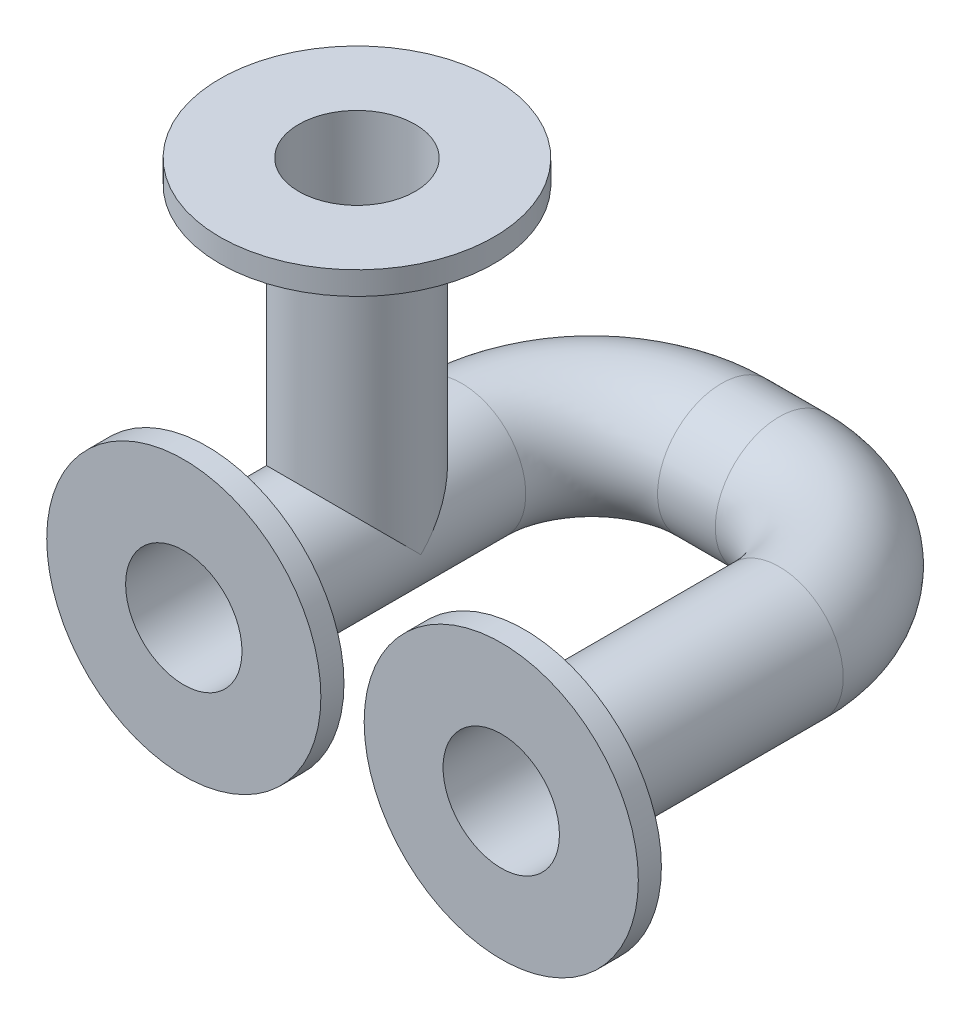
from build123d import *
from build123d.topology import SkipClean

# Parameters (mm, degrees)
SKETCH1_R           = 66.5
SKETCH1_R_2         = 60.5
SKETCH3_R           = 142.5
SKETCH3_R_2         = 60.5
BOSS_EXTRUDE1_DEPTH = 24
SKETCH4_R           = 66.5
SKETCH4_R_2         = 60.5
BOSS_EXTRUDE2_DEPTH = 300
SKETCH5_R           = 142.5
SKETCH5_R_2         = 60.5
BOSS_EXTRUDE3_DEPTH = 24


with BuildPart() as part:
    # Sweep1: sweep along a path in Sketch2
    with BuildLine(Plane(origin=(0, 0, 0), x_dir=(1, 0, 0), z_dir=(0, 1, 0))) as sweep1_path:
        Line((0, 0), (0, 265))
        ThreePointArc((0, 265), (39.54058454, 360.45941546), (135, 400))
        Line((135, 400), (195, 400))
        ThreePointArc((195, 400), (290.45941546, 360.45941546), (330, 265))
        Line((330, 265), (330, 0))
    # Sketch1 → Sweep1 (sweep)
    with BuildSketch(Plane.XY):
        Circle(SKETCH1_R)
        Circle(SKETCH1_R_2, mode=Mode.SUBTRACT)
    sweep(path=sweep1_path.line)

    # Sketch3 → Boss-Extrude1 (add)
    # profile 1 of 2: a face of its own
    with SkipClean():  # the faces are left unmerged after this step: merging them gives an invalid solid
        with BuildSketch(Plane.XY):
            with Locations((330, 0)):
                Circle(SKETCH3_R)
            with Locations((330, 0)):
                Circle(SKETCH3_R_2, mode=Mode.SUBTRACT)
        # profile 2 of 2: a face of its own
        with BuildSketch(Plane.XY):
            Circle(SKETCH3_R)
            with Locations(Location((0, 0, 0), (0, 0, 180))):
                Circle(SKETCH3_R_2, mode=Mode.SUBTRACT)
        extrude(amount=BOSS_EXTRUDE1_DEPTH)

    # Sketch4 → Boss-Extrude2 (add)
    with SkipClean():  # the faces are left unmerged after this step: merging them gives an invalid solid
        with BuildSketch(Plane(origin=(0, 0, 0), x_dir=(1, 0, 0), z_dir=(0, 1, 0))):
            with Locations((0, 156)):
                Circle(SKETCH4_R)
            with Locations(Location((0, 156, 0), (0, 0, 90))):
                Circle(SKETCH4_R_2, mode=Mode.SUBTRACT)
        extrude(amount=BOSS_EXTRUDE2_DEPTH)

    # Sketch5 → Boss-Extrude3 (add)
    with SkipClean():  # the faces are left unmerged after this step: merging them gives an invalid solid
        with BuildSketch(Plane(origin=(0, 300, 0), x_dir=(1, 0, 0), z_dir=(0, 1, 0))):
            with Locations(Location((0, 156, 0), (0, 0, 270))):
                Circle(SKETCH5_R)
            with Locations(Location((0, 156, 0), (0, 0, 90))):
                Circle(SKETCH5_R_2, mode=Mode.SUBTRACT)
        extrude(amount=BOSS_EXTRUDE3_DEPTH)


solid = part.part
